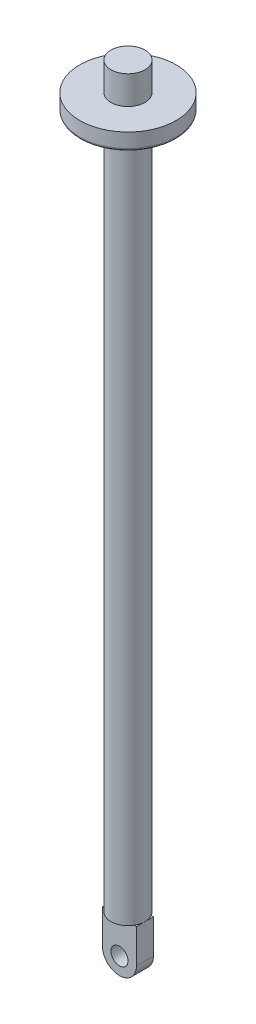
from build123d import *

# Parameters (mm, degrees)
SKETCH1_R           = 3
BOSS_EXTRUDE1_DEPTH = 130
SKETCH2_R           = 3
SKETCH2_R_2         = 1.5
BOSS_EXTRUDE2_DEPTH = 1.5
SKETCH3_R           = 8.5
BOSS_EXTRUDE3_DEPTH = 3
FILLET1_R           = 0.5


with BuildPart() as part:
    # Sketch1 → Boss-Extrude1 (new body)
    with BuildSketch(Plane(origin=(0, 0, 0), x_dir=(1, 0, 0), z_dir=(0, 1, 0))):
        with Locations(Location((0, 0, 0), (0, 0, 270))):
            Circle(SKETCH1_R)
    extrude(amount=BOSS_EXTRUDE1_DEPTH)

    # Sketch2 → Boss-Extrude2 (add, symmetric)
    # profile 1 of 2: a face of its own
    with BuildSketch(Plane.XY):
        with BuildLine():
            Line((3, 0), (-3, 0))
            Line((-3, 0), (-3, -6))
            ThreePointArc((-3, -6), (0, -3), (3, -6))
            Line((3, -6), (3, 0))
        make_face()
    # profile 2 of 2: a face of its own
    with BuildSketch(Plane.XY):
        with Locations((0, -6)):
            Circle(SKETCH2_R)
        with Locations((0, -6)):
            Circle(SKETCH2_R_2, mode=Mode.SUBTRACT)
    extrude(amount=BOSS_EXTRUDE2_DEPTH, both=True)

    # Sketch3 → Boss-Extrude3 (add)
    with BuildSketch(Plane(origin=(0, 122, 0), x_dir=(1, 0, 0), z_dir=(0, 1, 0))):
        with Locations(Location((0, 0, 0), (0, 0, 270))):
            Circle(SKETCH3_R)
    extrude(amount=BOSS_EXTRUDE3_DEPTH)

    # Fillet1
    fillet1_edges = [part.edges().sort_by_distance(p)[0] for p in [
        (0, 122, -8.5),
    ]]
    fillet(fillet1_edges, radius=FILLET1_R)


solid = part.part
